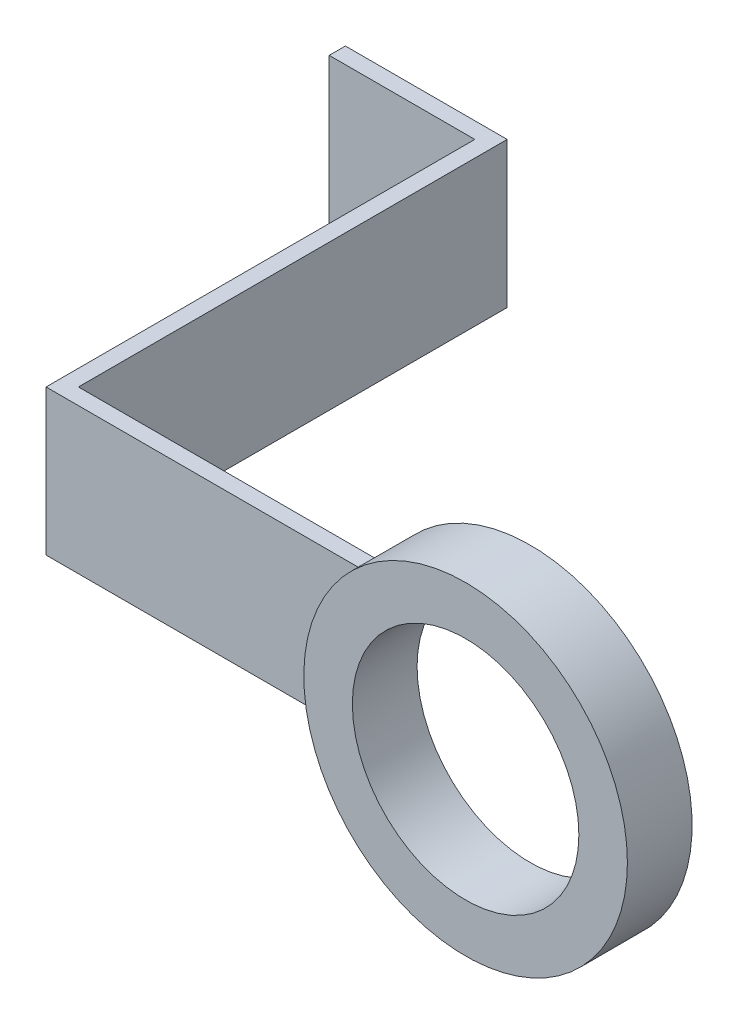
from build123d import *

# Parameters (mm, degrees)
SKETCH_1_R      = 20
SKETCH_1_R_2    = 14
EXTRUDE_1_DEPTH = 4
SKETCH_2_W      = 40
SKETCH_2_H      = 18
EXTRUDE_2_DEPTH = 2
SKETCH_3_W      = 2
SKETCH_3_H      = 18
EXTRUDE_3_DEPTH = 53
SKETCH_4_W      = 2
SKETCH_4_H      = 18
EXTRUDE_4_DEPTH = 18


with BuildPart() as part:
    # 草图1 → 凸台-拉伸1 (new, symmetric)
    with BuildSketch(Plane.XY):
        Circle(SKETCH_1_R)
        Circle(SKETCH_1_R_2, mode=Mode.SUBTRACT)
    extrude(amount=EXTRUDE_1_DEPTH, both=True)

    # 草图2 → 凸台-拉伸2 (add)
    with BuildSketch(Plane(origin=(0, 0, -4), x_dir=(-1, 0, 0), z_dir=(0, 0, -1))):
        with Locations((37.860571099, 0)):
            Rectangle(SKETCH_2_W, SKETCH_2_H)
    extrude(amount=-EXTRUDE_2_DEPTH)

    # 草图3 → 凸台-拉伸3 (add)
    with BuildSketch(Plane(origin=(0, 0, -4), x_dir=(-1, 0, 0), z_dir=(0, 0, -1))):
        with Locations((56.860571099, 0)):
            Rectangle(SKETCH_3_W, SKETCH_3_H)
    extrude(amount=EXTRUDE_3_DEPTH)

    # 草图4 → 凸台-拉伸4 (add)
    with BuildSketch(Plane.ZY.offset(57.860571099)):
        with Locations((-56, 0)):
            Rectangle(SKETCH_4_W, SKETCH_4_H)
    extrude(amount=EXTRUDE_4_DEPTH)


solid = part.part
